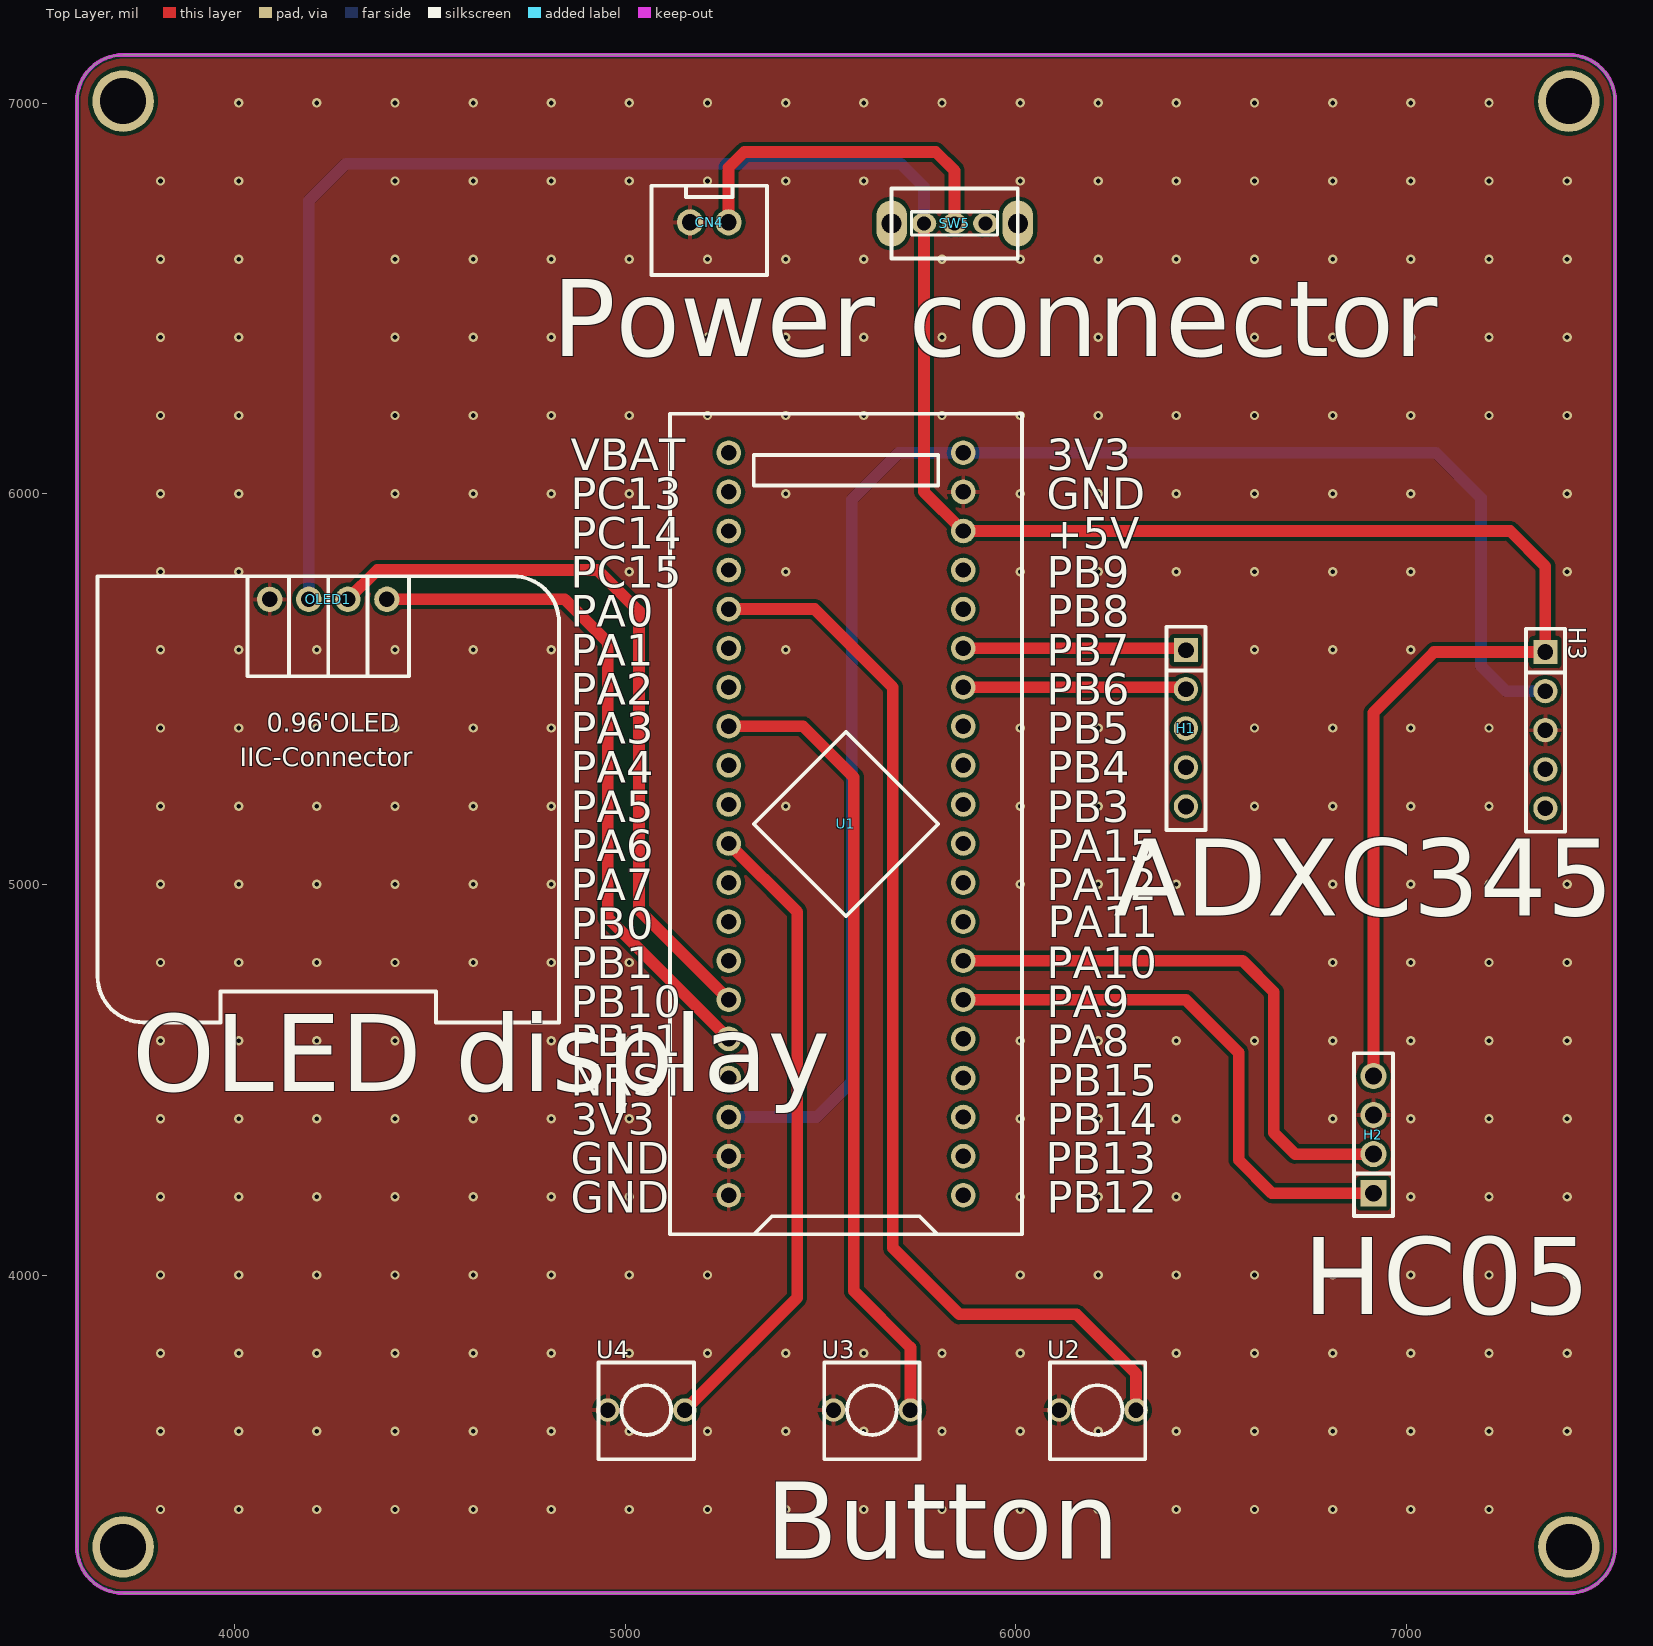
[diagram p0: Top Layer view]
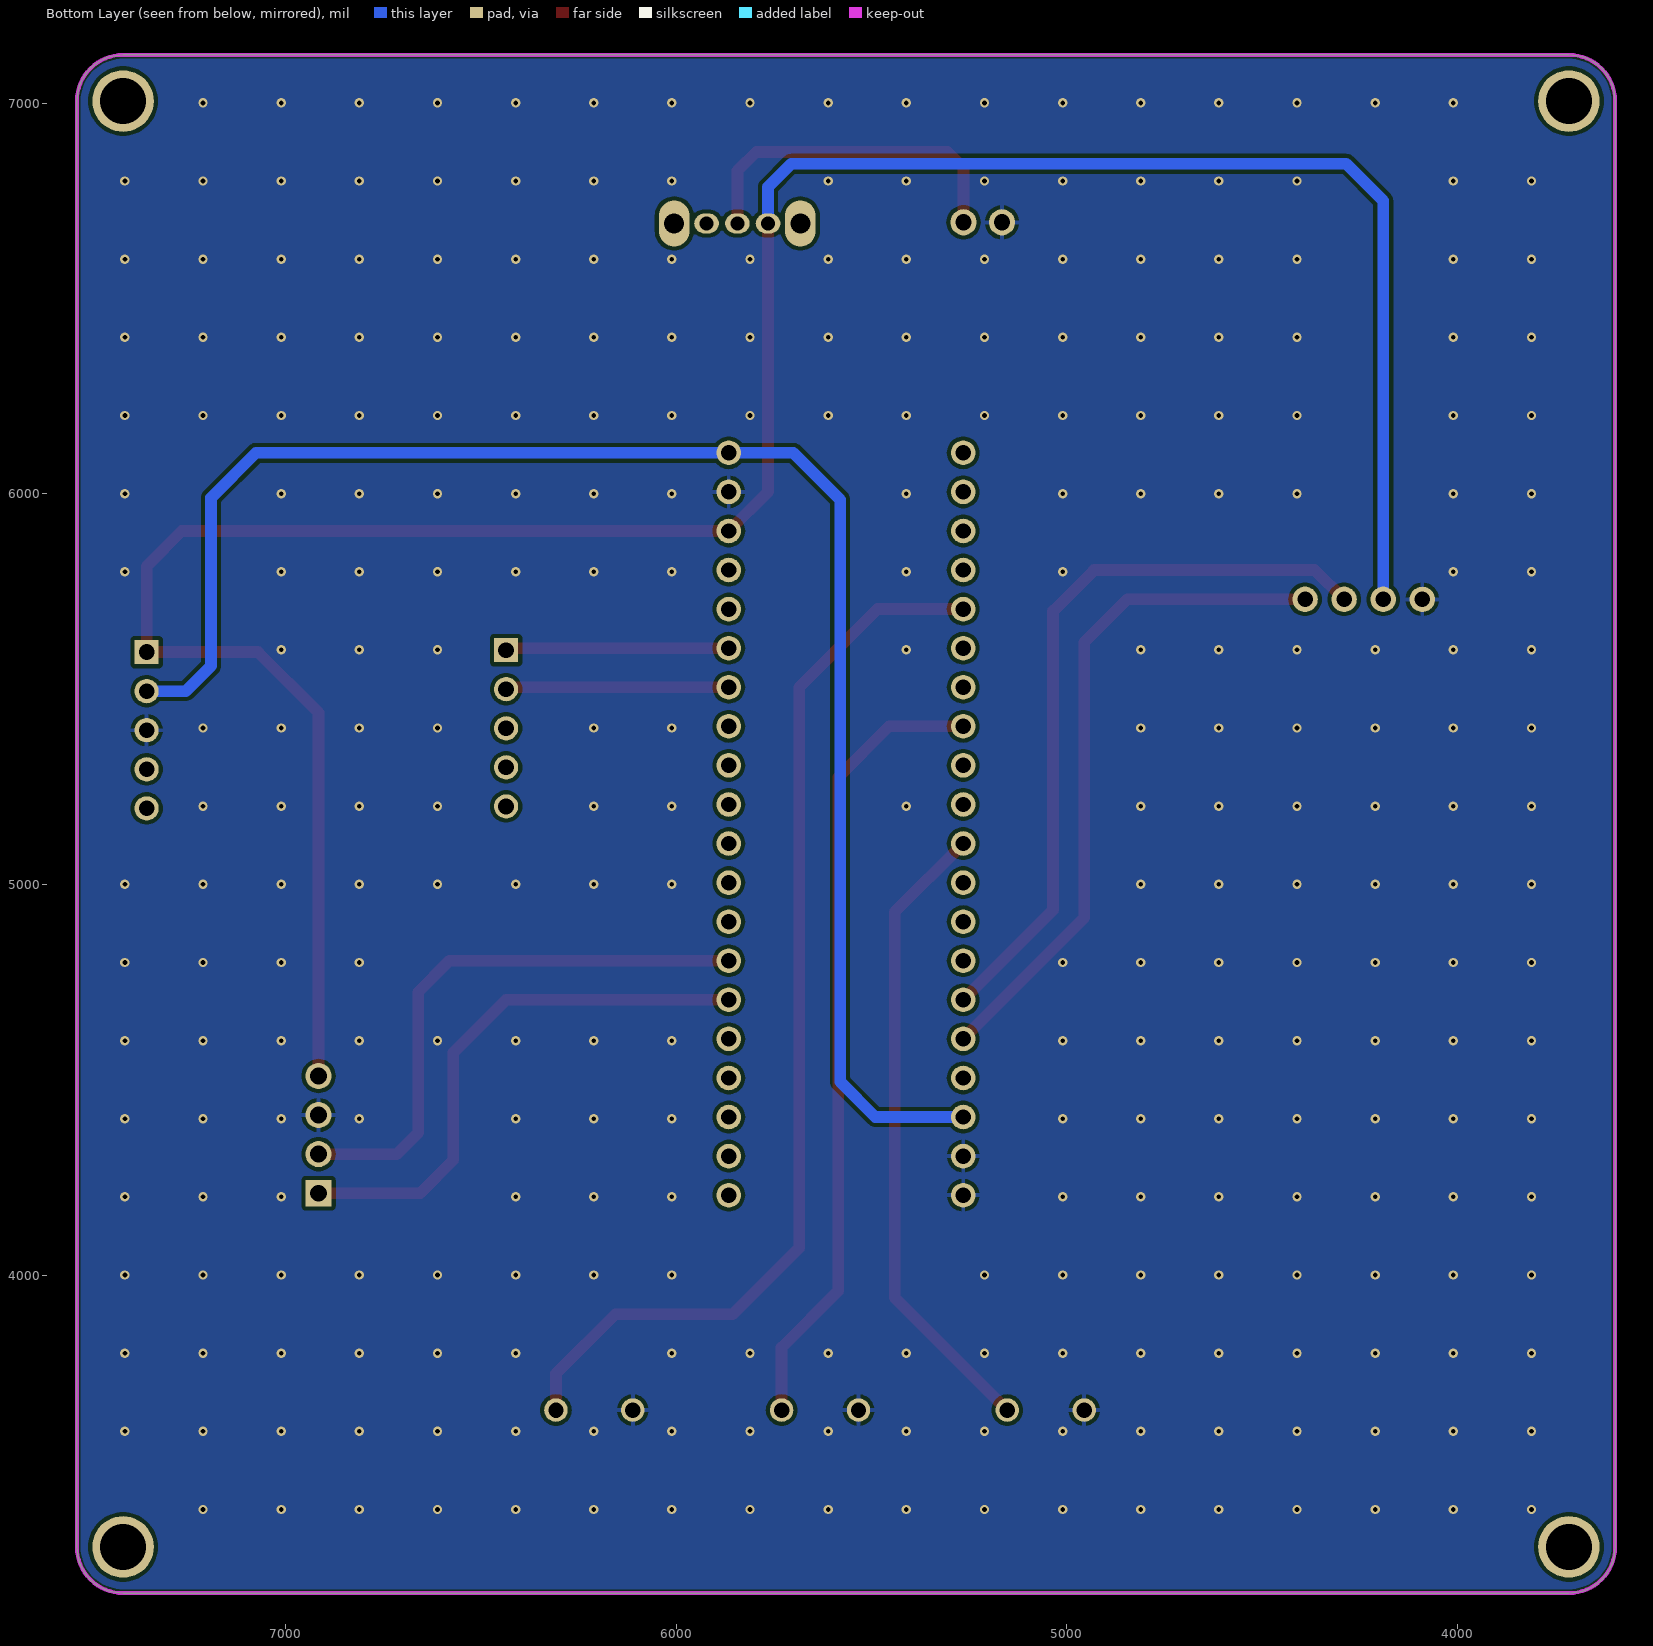
[diagram p1: Bottom Layer view, seen from below]
# Altium PCB MISC51878.pcbdoc
Units mil, origin at the board's own origin, x right, y up, seen from the top; angles counter-clockwise.
Board outline 3937.01 x 3937.01 mil, 2 copper layers (Top Layer, Bottom Layer), stack 62.206 mil thick; 10 components, 38 nets, 75 pads, 286 vias.

## Layer stack, top to bottom
Top Solder Mask Layer: solder mask 0.394, Dk 3.3
Top Layer: signal copper 1.379
Dielectric1: surface 59.449, FR4, Dk 4.5
Bottom Layer: signal copper 1.378
Bottom Solder Mask Layer: solder mask 0.394, Dk 3.3

## Board outline
3714.61,7123.5 ccw(c3714.61,7005.39) 3596.5,7005.39 3596.5,3304.61 ccw(c3714.61,3304.61) 3714.61,3186.5 7415.39,3186.5 ccw(c7415.39,3304.61) 7533.5,3304.61 7533.5,7005.39 ccw(c7415.39,7005.39) 7415.39,7123.5 3714.61,7123.5

## Design rules (kind name [scope] priority, off if disabled: settings)
BoardOutlineClearance copperThickness2oz_1 [All] p2 off: genericclearance=7.99 ignorepadtopadclearanceinfootprint=FALSE except(0: Arc-SplitContinuation Track-SplitContinuation SMDPad-SplitContinuation THPad-SplitContinuation Via-SplitContinuation Fill-SplitContinuation Region-SplitContinuation Poly-SplitContinuation Text-SplitContinuation Hole-SplitContinuation; 5.98: Arc-CutoutEdge Track-CutoutEdge SMDPad-CutoutEdge THPad-CutoutEdge Via-CutoutEdge Text-CutoutEdge; 6.9: Hole-OutlineEdge Hole-CutoutEdge; 10: Poly-OutlineEdge Poly-CutoutEdge; 11.81: Arc-OutlineEdge Track-OutlineEdge SMDPad-OutlineEdge THPad-OutlineEdge Via-OutlineEdge Fill-OutlineEdge Region-OutlineEdge Text-OutlineEdge Fill-CutoutEdge Region-CutoutEdge)
BoardOutlineClearance Plane_innerPlane_1 [All] p4 off: genericclearance=4.02 ignorepadtopadclearanceinfootprint=FALSE except(0: Arc-SplitContinuation Track-SplitContinuation SMDPad-SplitContinuation THPad-SplitContinuation Via-SplitContinuation Fill-SplitContinuation Region-SplitContinuation Poly-SplitContinuation Text-SplitContinuation Hole-SplitContinuation; 5.98: Arc-CutoutEdge Track-CutoutEdge SMDPad-CutoutEdge THPad-CutoutEdge Via-CutoutEdge Text-CutoutEdge; 6.9: Hole-OutlineEdge Hole-CutoutEdge; 10: Poly-OutlineEdge Poly-CutoutEdge; 11.81: Arc-OutlineEdge Track-OutlineEdge SMDPad-OutlineEdge THPad-OutlineEdge Via-OutlineEdge Fill-OutlineEdge Region-OutlineEdge Text-OutlineEdge Fill-CutoutEdge Region-CutoutEdge)
BoardOutlineClearance Copper_copperRegion_1 [All] p6 off: genericclearance=4.02 ignorepadtopadclearanceinfootprint=FALSE except(0: Arc-SplitContinuation Track-SplitContinuation SMDPad-SplitContinuation THPad-SplitContinuation Via-SplitContinuation Fill-SplitContinuation Region-SplitContinuation Poly-SplitContinuation Text-SplitContinuation Hole-SplitContinuation; 5.98: Arc-CutoutEdge Track-CutoutEdge SMDPad-CutoutEdge THPad-CutoutEdge Via-CutoutEdge Text-CutoutEdge; 6.9: Hole-OutlineEdge Hole-CutoutEdge; 10: Poly-OutlineEdge Poly-CutoutEdge; 11.81: Arc-OutlineEdge Track-OutlineEdge SMDPad-OutlineEdge THPad-OutlineEdge Via-OutlineEdge Fill-OutlineEdge Region-OutlineEdge Text-OutlineEdge Fill-CutoutEdge Region-CutoutEdge)
BoardOutlineClearance Copper_copperRegion_copperThickness1oz_1 [All] p8 off: genericclearance=4.02 ignorepadtopadclearanceinfootprint=FALSE except(0: Arc-SplitContinuation Track-SplitContinuation SMDPad-SplitContinuation THPad-SplitContinuation Via-SplitContinuation Fill-SplitContinuation Region-SplitContinuation Poly-SplitContinuation Text-SplitContinuation Hole-SplitContinuation; 5.98: Arc-CutoutEdge Track-CutoutEdge SMDPad-CutoutEdge THPad-CutoutEdge Via-CutoutEdge Text-CutoutEdge; 6.9: Hole-OutlineEdge Hole-CutoutEdge; 10: Poly-OutlineEdge Poly-CutoutEdge; 11.81: Arc-OutlineEdge Track-OutlineEdge SMDPad-OutlineEdge THPad-OutlineEdge Via-OutlineEdge Fill-OutlineEdge Region-OutlineEdge Text-OutlineEdge Fill-CutoutEdge Region-CutoutEdge)
BoardOutlineClearance Copper_copperRegion_Copper_copperRegion_1 [All] p10 off: genericclearance=4.02 ignorepadtopadclearanceinfootprint=FALSE except(0: Arc-SplitContinuation Track-SplitContinuation SMDPad-SplitContinuation THPad-SplitContinuation Via-SplitContinuation Fill-SplitContinuation Region-SplitContinuation Poly-SplitContinuation Text-SplitContinuation Hole-SplitContinuation; 5.98: Arc-CutoutEdge Track-CutoutEdge SMDPad-CutoutEdge THPad-CutoutEdge Via-CutoutEdge Text-CutoutEdge; 6.9: Hole-OutlineEdge Hole-CutoutEdge; 10: Poly-OutlineEdge Poly-CutoutEdge; 11.81: Arc-OutlineEdge Track-OutlineEdge SMDPad-OutlineEdge THPad-OutlineEdge Via-OutlineEdge Fill-OutlineEdge Region-OutlineEdge Text-OutlineEdge Fill-CutoutEdge Region-CutoutEdge)
BoardOutlineClearance copperThickness1oz_1 [All] p12: genericclearance=4.02 ignorepadtopadclearanceinfootprint=FALSE except(0: Arc-SplitContinuation Track-SplitContinuation SMDPad-SplitContinuation THPad-SplitContinuation Via-SplitContinuation Fill-SplitContinuation Region-SplitContinuation Poly-SplitContinuation Text-SplitContinuation Hole-SplitContinuation; 5.98: Arc-CutoutEdge Track-CutoutEdge SMDPad-CutoutEdge THPad-CutoutEdge Via-CutoutEdge Text-CutoutEdge; 6.9: Hole-OutlineEdge Hole-CutoutEdge; 10: Poly-OutlineEdge Poly-CutoutEdge; 11.81: Arc-OutlineEdge Track-OutlineEdge SMDPad-OutlineEdge THPad-OutlineEdge Via-OutlineEdge Fill-OutlineEdge Region-OutlineEdge Text-OutlineEdge Fill-CutoutEdge Region-CutoutEdge)
Clearance copperThickness2oz [All] p1 off: gap=7.99 ignorepadtopadclearanceinfootprint=FALSE except(5.98: SMDPad-Track SMDPad-SMDPad THPad-Track SMDPad-THPad THPad-THPad Track-Via SMDPad-Via THPad-Via Via-Via Fill-SMDPad Region-SMDPad Fill-THPad Region-THPad Fill-Via Region-Via Fill-Fill Fill-Region Region-Region Arc-Track Arc-SMDPad Arc-THPad Arc-Via Fill-Arc Region-Arc Arc-Arc Text-Track SMDPad-Text Text-THPad Text-Via Fill-Text Region-Text Arc-Text Text-Text; 6.9: Hole-Track Hole-SMDPad Hole-THPad Hole-Via Fill-Hole Region-Hole Hole-Arc Hole-Text; 10: Poly-Track Poly-SMDPad Poly-THPad Poly-Via Poly-Fill Poly-Region Poly-Poly Poly-Arc Poly-Text Poly-Hole; 11.81: Fill-Track Region-Track)
Clearance Plane_innerPlane [All] p3 off: gap=4.02 ignorepadtopadclearanceinfootprint=FALSE except(5.98: SMDPad-Track SMDPad-SMDPad THPad-Track SMDPad-THPad THPad-THPad Track-Via SMDPad-Via THPad-Via Via-Via Fill-SMDPad Region-SMDPad Fill-THPad Region-THPad Fill-Via Region-Via Fill-Fill Fill-Region Region-Region Arc-Track Arc-SMDPad Arc-THPad Arc-Via Fill-Arc Region-Arc Arc-Arc Text-Track SMDPad-Text Text-THPad Text-Via Fill-Text Region-Text Arc-Text Text-Text; 6.9: Hole-Track Hole-SMDPad Hole-THPad Hole-Via Fill-Hole Region-Hole Hole-Arc Hole-Text; 10: Poly-Track Poly-SMDPad Poly-THPad Poly-Via Poly-Fill Poly-Region Poly-Poly Poly-Arc Poly-Text Poly-Hole; 11.81: Fill-Track Region-Track)
Clearance Copper_copperRegion [All] p5 off: gap=4.02 ignorepadtopadclearanceinfootprint=FALSE except(5.98: SMDPad-Track SMDPad-SMDPad THPad-Track SMDPad-THPad THPad-THPad Track-Via SMDPad-Via THPad-Via Via-Via Fill-SMDPad Region-SMDPad Fill-THPad Region-THPad Fill-Via Region-Via Fill-Fill Fill-Region Region-Region Arc-Track Arc-SMDPad Arc-THPad Arc-Via Fill-Arc Region-Arc Arc-Arc Text-Track SMDPad-Text Text-THPad Text-Via Fill-Text Region-Text Arc-Text Text-Text; 6.9: Hole-Track Hole-SMDPad Hole-THPad Hole-Via Fill-Hole Region-Hole Hole-Arc Hole-Text; 10: Poly-Track Poly-SMDPad Poly-THPad Poly-Via Poly-Fill Poly-Region Poly-Poly Poly-Arc Poly-Text Poly-Hole; 11.81: Fill-Track Region-Track)
Clearance Copper_copperRegion_copperThickness1oz [All] p7 off: gap=4.02 ignorepadtopadclearanceinfootprint=FALSE except(5.98: SMDPad-Track SMDPad-SMDPad THPad-Track SMDPad-THPad THPad-THPad Track-Via SMDPad-Via THPad-Via Via-Via Fill-SMDPad Region-SMDPad Fill-THPad Region-THPad Fill-Via Region-Via Fill-Fill Fill-Region Region-Region Arc-Track Arc-SMDPad Arc-THPad Arc-Via Fill-Arc Region-Arc Arc-Arc Text-Track SMDPad-Text Text-THPad Text-Via Fill-Text Region-Text Arc-Text Text-Text; 6.9: Hole-Track Hole-SMDPad Hole-THPad Hole-Via Fill-Hole Region-Hole Hole-Arc Hole-Text; 10: Poly-Track Poly-SMDPad Poly-THPad Poly-Via Poly-Fill Poly-Region Poly-Poly Poly-Arc Poly-Text Poly-Hole; 11.81: Fill-Track Region-Track)
Clearance Copper_copperRegion_Copper_copperRegion [All] p9 off: gap=4.02 ignorepadtopadclearanceinfootprint=FALSE except(5.98: SMDPad-Track SMDPad-SMDPad THPad-Track SMDPad-THPad THPad-THPad Track-Via SMDPad-Via THPad-Via Via-Via Fill-SMDPad Region-SMDPad Fill-THPad Region-THPad Fill-Via Region-Via Fill-Fill Fill-Region Region-Region Arc-Track Arc-SMDPad Arc-THPad Arc-Via Fill-Arc Region-Arc Arc-Arc Text-Track SMDPad-Text Text-THPad Text-Via Fill-Text Region-Text Arc-Text Text-Text; 6.9: Hole-Track Hole-SMDPad Hole-THPad Hole-Via Fill-Hole Region-Hole Hole-Arc Hole-Text; 10: Poly-Track Poly-SMDPad Poly-THPad Poly-Via Poly-Fill Poly-Region Poly-Poly Poly-Arc Poly-Text Poly-Hole; 11.81: Fill-Track Region-Track)
Clearance copperThickness1oz [All] p11: gap=4.02 ignorepadtopadclearanceinfootprint=FALSE except(5.98: SMDPad-Track SMDPad-SMDPad THPad-Track SMDPad-THPad THPad-THPad Track-Via SMDPad-Via THPad-Via Via-Via Fill-SMDPad Region-SMDPad Fill-THPad Region-THPad Fill-Via Region-Via Fill-Fill Fill-Region Region-Region Arc-Track Arc-SMDPad Arc-THPad Arc-Via Fill-Arc Region-Arc Arc-Arc Text-Track SMDPad-Text Text-THPad Text-Via Fill-Text Region-Text Arc-Text Text-Text; 6.9: Hole-Track Hole-SMDPad Hole-THPad Hole-Via Fill-Hole Region-Hole Hole-Arc Hole-Text; 10: Poly-Track Poly-SMDPad Poly-THPad Poly-Via Poly-Fill Poly-Region Poly-Poly Poly-Arc Poly-Text Poly-Hole; 11.81: Fill-Track Region-Track)
DiffPairsRouting differentialPair [All] p1: maxlimit=6 minlimit=6 mostfreqgap=6 toplayer_minwidth=5 toplayer_prefwidth=10 toplayer_maxwidth=100 toplayer_mingap=6 toplayer_prefgap=6 toplayer_maxgap=6 bottomlayer_minwidth=5 bottomlayer_prefwidth=10 bottomlayer_maxwidth=100 bottomlayer_mingap=6 bottomlayer_prefgap=6 bottomlayer_maxgap=6 maxuncoupledlength=10
HoleToHoleClearance otherClearance [All] p1: gap=11.81 allowstackedmicrovias=TRUE
Length netLength [All] p1: minlimit=0 maxlimit=0
PasteMaskExpansion pasteMaskExpansion [All] p1: expansion=0
PlaneConnect innerPlane [All] p1: planeconnectstyle=Relief reliefexpansion=20 reliefentries=4 reliefconductorwidth=10 reliefairgap=10
PolygonConnect copperRegion_copperThickness1oz [All] p1 off: connectstyle=Relief reliefconductorwidth=10 reliefentries=4 polygonreliefangle="90 Angle" airgapwidth=10 via.connectstyle=Relief via.reliefconductorwidth=10 via.reliefentries=4 via.polygonreliefangle="90 Angle" via.airgapwidth=10
PolygonConnect copperRegion_Copper_copperRegion [All] p2 off: connectstyle=Relief reliefconductorwidth=10 reliefentries=4 polygonreliefangle="90 Angle" airgapwidth=10 via.connectstyle=Relief via.reliefconductorwidth=10 via.reliefentries=4 via.polygonreliefangle="90 Angle" via.airgapwidth=10
PolygonConnect copperRegion [All] p3: connectstyle=Relief reliefconductorwidth=10 reliefentries=4 polygonreliefangle="90 Angle" airgapwidth=10 via.connectstyle=Relief via.reliefconductorwidth=10 via.reliefentries=4 via.polygonreliefangle="90 Angle" via.airgapwidth=10
RoutingVias viaSize [All] p1: holewidth=12.01 width=24.02 viastyle="Through Hole" minholewidth=11.81 minwidth=19.68 maxholewidth=248.03 maxwidth=393.7
SolderMaskExpansion solderMaskExpansion [IsVia] p1: expansion=-1000 istentingtop=TRUE
SolderMaskExpansion solderMaskExpansion [All] p2: expansion=2 istentingtop=FALSE
Width copperThickness2oz_2 [All] p1 off: maxlimit=100 minlimit=8 preferedwidth=10
Width copperThickness1oz_2 [All] p2: maxlimit=100 minlimit=5 preferedwidth=10

## Components (designator, comment, footprint, x,y, rotation, side; value= is the part's Value field where it differs from the comment)
CN4 "XH2.54*2P_through-hole" CONN-TH_2P-P2.50-XH2.54-2P 5215,6695 r0 top
H1 "" HDR-TH_5P-P2.54-V-F 6435,5400 r270 top
H2 "" HDR-TH_4P-P2.54-V-F 6915,4360 r90 top
H3 "" HDR-TH_5P-P2.54-V-F 7355,5395 r270 top
OLED1 "" 0.96OLED_4P 4240,5730 r0 top
SW5 "" 拨动开关 5837.9,6692.05 r0 top
U1 "STM32F103C8T6-Card" CONN-TH_L53.3-W22.9_STM32F103C8T6-CARD 5565,5155 r90 top
U2 "TL59BF160Q" KEY-TH_L6.2-W6.2-P5.00 6208.93,3655 r0 top
U3 "TL59BF160Q" KEY-TH_L6.2-W6.2-P5.00 5631.43,3655 r0 top
U4 "TL59BF160Q" KEY-TH_L6.2-W6.2-P5.00 5053.93,3655 r0 top

## Footprints (in the part's own frame and the unit in brackets; to place one, negate y for a bottom-side part, rotate by r counter-clockwise, add the part's x,y. Pads: shape width x height; smd on the part's side, far side on the other; paste and mask are expansions set on the pad)
0.96OLED_4P [mm]
  round 1.65 hole 1 copper offset 0,0: 1(-3.81,-0.001) 2(-1.27,0.002) 3(1.27,0.002) 4(3.81,0.002)
  silkscreen extent -15,-27.5 15,1.5
CONN-TH_2P-P2.50-XH2.54-2P [mm]
  round 1.7 hole 1.05 paste+0 mask+0.05: 1(1.25,0) 2(-1.25,0)
  silkscreen extent -3.75,-3.42 3.75,2.37
CONN-TH_L53.3-W22.9_STM32F103C8T6-CARD [mm]
  round 1.6 hole 1: 1(-24.13,-7.62) 2(-21.59,-7.62) 3(-19.05,-7.62) 4(-16.51,-7.62) 5(-13.97,-7.62) 6(-11.43,-7.62) 7(-8.89,-7.62) 8(-6.35,-7.62) 9(-3.81,-7.62) 10(-1.27,-7.62) 11(1.27,-7.62) 12(3.81,-7.62) 13(6.35,-7.62) 14(8.89,-7.62) 15(11.43,-7.62) 16(13.97,-7.62) 17(16.51,-7.62) 18(19.05,-7.62) 19(21.59,-7.62) 20(24.13,-7.62) 21(24.13,7.62) 22(21.59,7.62) 23(19.05,7.62) 24(16.51,7.62) 25(13.97,7.62) 26(11.43,7.62) 27(8.89,7.62) 28(6.35,7.62) 29(3.81,7.62) 30(1.27,7.62) 31(-1.27,7.62) 32(-3.81,7.62) 33(-6.35,7.62) 34(-8.89,7.62) 35(-11.43,7.62) 36(-13.97,7.62) 37(-16.51,7.62) 38(-19.05,7.62) 39(-21.59,7.62) 40(-24.13,7.62)
  silkscreen extent -26.67,-11.43 26.67,11.43
HDR-TH_4P-P2.54-V-F [mm]
  rect 1.7x1.7 hole 1.1: 1(-3.81,0)
  round 1.7 hole 1.1: 2(-1.27,0) 3(1.27,0) 4(3.81,0)
  silkscreen extent -5.29,-1.27 5.29,1.27
HDR-TH_5P-P2.54-V-F [mil]
  rect 62x62 hole 40.16: 1(-200,0)
  round 62 hole 40.16: 2(-100,0) 3(0,0) 4(100,0) 5(200,0)
  silkscreen extent -260,-50 260,50
KEY-TH_L6.2-W6.2-P5.00 [mil]
  round 60 hole 39.37: 1(-98.43,0) 2(98.42,0)
  silkscreen extent -122,-126 122,122
拨动开关 [mil]
  oval 63x51.2 hole 35.4 paste+0 mask+2: 1(-73.4,0) 2(5,0) 3(84,0)
  oval 78.7x118.1 hole 51.2 paste+0 mask+2: 4(166.7,0) 5(-156.1,0)
  silkscreen extent -156,-90 167,90

## Free pads (board coordinates)
  round 157.48 hole 118.11: 1(3714.61,7005.39) 1(3714.61,3304.61) 1(7415.39,7005.39) 1(7415.39,3304.61)

## Via types
v1: diameter 24.02, hole 12, Top Layer to Bottom Layer, 286 vias

## Nets (pads, with @x,y where several pads share a name; then routed paths per layer and width w, separated by ;. In a path a pad name is that pad's centre, name@x,y a point inside that pad or via, vN(x,y) a via of type N, cw(c..) or ccw(c..) an arc to the next point about the centre after c; other vN are vias at no path point)
$1N17118: CN4.1 SW5.2 | length 889.7
  Top Layer w30: CN4.1 5264.22,6834.22 5305,6875 5795,6875 5842.9,6827.1 SW5.2
+5V: H2.4 H3.1 OLED1.2 SW5.1 U1.18 | length 6762.1
  Top Layer w30: SW5.1 5764.5,6005.5 U1.18 7265,5905 7355,5815 H3.1 7070,5595 6915,5440 H2.4
  Bottom Layer w30: OLED1.2@4190,5730.05 4190,6750 4285,6845 5705,6845 5764.5,6785.5 SW5.1
GND: CN4.2 H2.3 H3.3 OLED1.1 U1.19 U1.39 U1.40 U2.1 U3.1 U4.1
  other v1: 3810.6,3400.6 4010.6,3400.6 4210.6,3400.6 4410.6,3400.6 4610.6,3400.6 4810.6,3400.6 5010.6,3400.6 5210.6,3400.6 5410.6,3400.6 5610.6,3400.6 5810.6,3400.6 6010.6,3400.6 6210.6,3400.6 6410.6,3400.6 6610.6,3400.6 6810.6,3400.6 7010.6,3400.6 7210.6,3400.6 3810.6,3600.6 4010.6,3600.6 4210.6,3600.6 4410.6,3600.6 4610.6,3600.6 4810.6,3600.6 5010.6,3600.6 5210.6,3600.6 5410.6,3600.6 5610.6,3600.6 5810.6,3600.6 6010.6,3600.6 6210.6,3600.6 6410.6,3600.6 6610.6,3600.6 6810.6,3600.6 7010.6,3600.6 7210.6,3600.6 7410.6,3600.6 3810.6,3800.6 4010.6,3800.6 4210.6,3800.6 4410.6,3800.6 4610.6,3800.6 4810.6,3800.6 5010.6,3800.6 5210.6,3800.6 5410.6,3800.6 5610.6,3800.6 5810.6,3800.6 6010.6,3800.6 6410.6,3800.6 6610.6,3800.6 6810.6,3800.6 7010.6,3800.6 7210.6,3800.6 7410.6,3800.6 3810.6,4000.6 4010.6,4000.6 4210.6,4000.6 4410.6,4000.6 4610.6,4000.6 4810.6,4000.6 5010.6,4000.6 5210.6,4000.6 6010.6,4000.6 6210.6,4000.6 6410.6,4000.6 6610.6,4000.6 6810.6,4000.6 7010.6,4000.6 7210.6,4000.6 7410.6,4000.6 3810.6,4200.6 4010.6,4200.6 4210.6,4200.6 4410.6,4200.6 4610.6,4200.6 4810.6,4200.6 5010.6,4200.6 6010.6,4200.6 6210.6,4200.6 6410.6,4200.6 7010.6,4200.6 7210.6,4200.6 7410.6,4200.6 3810.6,4400.6 4010.6,4400.6 4210.6,4400.6 4410.6,4400.6 4610.6,4400.6 4810.6,4400.6 5010.6,4400.6 6010.6,4400.6 6210.6,4400.6 6410.6,4400.6 6810.6,4400.6 7010.6,4400.6 7210.6,4400.6 7410.6,4400.6 3810.6,4600.6 4010.6,4600.6 4210.6,4600.6 4410.6,4600.6 4610.6,4600.6 4810.6,4600.6 5010.6,4600.6 6010.6,4600.6 6210.6,4600.6 6410.6,4600.6 6610.6,4600.6 6810.6,4600.6 7010.6,4600.6 7210.6,4600.6 7410.6,4600.6 3810.6,4800.6 4010.6,4800.6 4210.6,4800.6 4410.6,4800.6 4610.6,4800.6 4810.6,4800.6 5010.6,4800.6 6810.6,4800.6 7010.6,4800.6 7210.6,4800.6 7410.6,4800.6 3810.6,5000.6 4010.6,5000.6 4210.6,5000.6 4410.6,5000.6 4610.6,5000.6 4810.6,5000.6 6010.6,5000.6 6210.6,5000.6 6410.6,5000.6 6610.6,5000.6 6810.6,5000.6 7010.6,5000.6 7210.6,5000.6 7410.6,5000.6 3810.6,5200.6 4010.6,5200.6 4210.6,5200.6 4410.6,5200.6 4610.6,5200.6 4810.6,5200.6 5410.6,5200.6 6010.6,5200.6 6210.6,5200.6 6610.6,5200.6 6810.6,5200.6 7010.6,5200.6 7210.6,5200.6 3810.6,5400.6 4010.6,5400.6 4210.6,5400.6 4410.6,5400.6 4610.6,5400.6 4810.6,5400.6 6010.6,5400.6 6210.6,5400.6 6610.6,5400.6 6810.6,5400.6 7010.6,5400.6 7210.6,5400.6 3810.6,5600.6 4010.6,5600.6 4210.6,5600.6 4410.6,5600.6 4610.6,5600.6 4810.6,5600.6 5410.6,5600.6 6610.6,5600.6 6810.6,5600.6 7010.6,5600.6 3810.6,5800.6 4010.6,5800.6 5010.6,5800.6 5410.6,5800.6 6010.6,5800.6 6210.6,5800.6 6410.6,5800.6 6610.6,5800.6 6810.6,5800.6 7010.6,5800.6 7410.6,5800.6 3810.6,6000.6 4010.6,6000.6 4410.6,6000.6 4610.6,6000.6 4810.6,6000.6 5010.6,6000.6 5410.6,6000.6 6010.6,6000.6 6210.6,6000.6 6410.6,6000.6 6610.6,6000.6 6810.6,6000.6 7010.6,6000.6 7410.6,6000.6 3810.6,6200.6 4010.6,6200.6 4410.6,6200.6 4610.6,6200.6 4810.6,6200.6 5010.6,6200.6 5210.6,6200.6 5410.6,6200.6 5610.6,6200.6 5810.6,6200.6 6010.6,6200.6 6210.6,6200.6 6410.6,6200.6 6610.6,6200.6 6810.6,6200.6 7010.6,6200.6 7210.6,6200.6 7410.6,6200.6 3810.6,6400.6 4010.6,6400.6 4410.6,6400.6 4610.6,6400.6 4810.6,6400.6 5010.6,6400.6 5210.6,6400.6 5410.6,6400.6 5610.6,6400.6 5810.6,6400.6 6010.6,6400.6 6210.6,6400.6 6410.6,6400.6 6610.6,6400.6 6810.6,6400.6 7010.6,6400.6 7210.6,6400.6 7410.6,6400.6 3810.6,6600.6 4010.6,6600.6 4410.6,6600.6 4610.6,6600.6 4810.6,6600.6 5010.6,6600.6 5210.6,6600.6 5410.6,6600.6 5610.6,6600.6 5810.6,6600.6 6010.6,6600.6 6210.6,6600.6 6410.6,6600.6 6610.6,6600.6 6810.6,6600.6 7010.6,6600.6 7210.6,6600.6 7410.6,6600.6 3810.6,6800.6 4010.6,6800.6 4410.6,6800.6 4610.6,6800.6 4810.6,6800.6 5010.6,6800.6 5210.6,6800.6 5410.6,6800.6 5610.6,6800.6 6010.6,6800.6 6210.6,6800.6 6410.6,6800.6 6610.6,6800.6 6810.6,6800.6 7010.6,6800.6 7210.6,6800.6 7410.6,6800.6 4010.6,7000.6 4210.6,7000.6 4410.6,7000.6 4610.6,7000.6 4810.6,7000.6 5010.6,7000.6 5210.6,7000.6 5410.6,7000.6 5610.6,7000.6 5810.6,7000.6 6010.6,7000.6 6210.6,7000.6 6410.6,7000.6 6610.6,7000.6 6810.6,7000.6 7010.6,7000.6 7210.6,7000.6
NRST: U1.37
PA0: U1.25 U2.2 | length 2786.4
  Top Layer w30: U1.25 5485,5705 5685,5505 5685,4070 5855,3900 6155,3900 6307.35,3747.64 U2.2
PA1: U1.26
PA2: U1.27
PA3: U1.28 U3.2 | length 2053.9
  Top Layer w30: U1.28 5455,5405 5585,5275 5585,3960 5729.85,3815.14 U3.2
PA4: U1.29
PA5: U1.30
PA6: U1.31 U4.2 | length 1641.6
  Top Layer w30: U4.2 5440,3942.64 5440,4930 U1.31
PA7: U1.32
PA8: U1.5
PA9: H2.1 U1.6 | length 1416.1
  Top Layer w30: U1.6 6435,4705 6570,4570 6570,4295 6655,4210 H2.1
PA10: H2.2 U1.7 | length 1465.9
  Top Layer w30: U1.7 6580,4805 6660,4725 6660,4365 6715,4310 H2.2
PA11: U1.8
PA12: U1.9
PA15: U1.10
PB0: U1.33
PB1: U1.34
PB3: U1.11
PB4: U1.12
PB5: U1.13
PB6: H1.2 U1.14 | length 572.1
  Top Layer w30: U1.14 6430,5505 H1.2
PB7: H1.1 U1.15 | length 572.1
  Top Layer w30: U1.15 6430,5605 H1.1
PB8: U1.16
PB9: U1.17
PB10: OLED1.3 U1.35 | length 1909.8
  Top Layer w30: OLED1.3@4290,5730.05 4364.95,5805 4930,5805 5035,5700 5035,4935 U1.35
PB11: OLED1.4 U1.36 | length 1754
  Top Layer w30: OLED1.4@4390,5730.05 4844.95,5730.05 4955,5620 4955,4915 U1.36
PB12: U1.1
PB13: U1.2
PB14: U1.3
PB15: U1.4
PC13: U1.22
PC14: U1.23
PC15: U1.24
VBAT: U1.21
VCC: H3.2 U1.20 U1.38 | length 4171.5
  Bottom Layer w30: U1.38 5490,4405 5580,4495 5580,5985 5700,6105 U1.20 7075,6105 7190,5990 7190,5560 7255,5495 H3.2
pads on no net: H1.3 H1.4 H1.5 H3.4 H3.5 SW5.3 SW5.4 SW5.5

## Polygon pours and split planes (outlines as drawn)
GND on Bottom Layer (solid, remove dead copper, pour order 2): 3525,7245 3525,3080 7700,3080 7700,7245
GND on Top Layer (solid, remove dead copper, pour order 2): 3000,7415 3000,3000 7930,3000 7930,7415

## Keep-outs
Board Outline Layer:
  the board outline again, w10

## Silkscreen, mask and mechanical layers (free items; w line width, h text height)
Top Silkscreen Layer:
  text "Power connector" at 4812.87,6351.57 h196.85
  text "VBAT" at 4860.95,6060 h80
  text "3V3" at 6079.16,6060 h80
  text "PC13" at 4860.95,5960 h80
  text "GND" at 6079.16,5960 h80
  text "PC14" at 4860.95,5860 h80
  text "+5V" at 6079.16,5860 h80
  text "PC15" at 4860.95,5760 h80
  text "PB9" at 6079.16,5760 h80
  text "PA0" at 4860.95,5660 h80
  text "PB8" at 6079.16,5660 h80
  text "PA1" at 4860.95,5560 h80
  text "PB7" at 6079.16,5560 h80
  text "PA2" at 4860.95,5460 h80
  text "PB6" at 6079.16,5460 h80
  text "PA3" at 4860.95,5360 h80
  text "PB5" at 6079.16,5360 h80
  text "PA4" at 4860.95,5260 h80
  text "PB4" at 6079.16,5260 h80
  text "PA5" at 4860.95,5160 h80
  text "PB3" at 6079.16,5160 h80
  text "PA6" at 4860.95,5060 h80
  text "PA15" at 6079.16,5060 h80
  text "PA7" at 4860.95,4960 h80
  text "PA12" at 6079.16,4960 h80
  text "ADXC345 sensor" at 6250,4920 h196.85
  text "PA11" at 6080.95,4865 h80
  text "PB0" at 4860.95,4860 h80
  text "PB1" at 4860.95,4760 h80
  text "PA10" at 6079.16,4760 h80
  text "PB10" at 4860.95,4660 h80
  text "PA9" at 6079.16,4660 h80
  text "PB11" at 4860.95,4560 h80
  text "PA8" at 6079.16,4560 h80
  text "OLED display" at 3738.66,4471.57 h196.85
  text "NRST" at 4860.95,4460 h80
  text "PB15" at 6079.16,4460 h80
  text "3V3" at 4860.95,4360 h80
  text "PB14" at 6079.16,4360 h80
  text "GND" at 4860.95,4260 h80
  text "PB13" at 6075.95,4260 h80
  text "GND" at 4860.95,4160 h80
  text "PB12" at 6079.16,4160 h80
  text "HC05" at 6735,3900 h196.85
  text "Button" at 5360,3275 h196.85